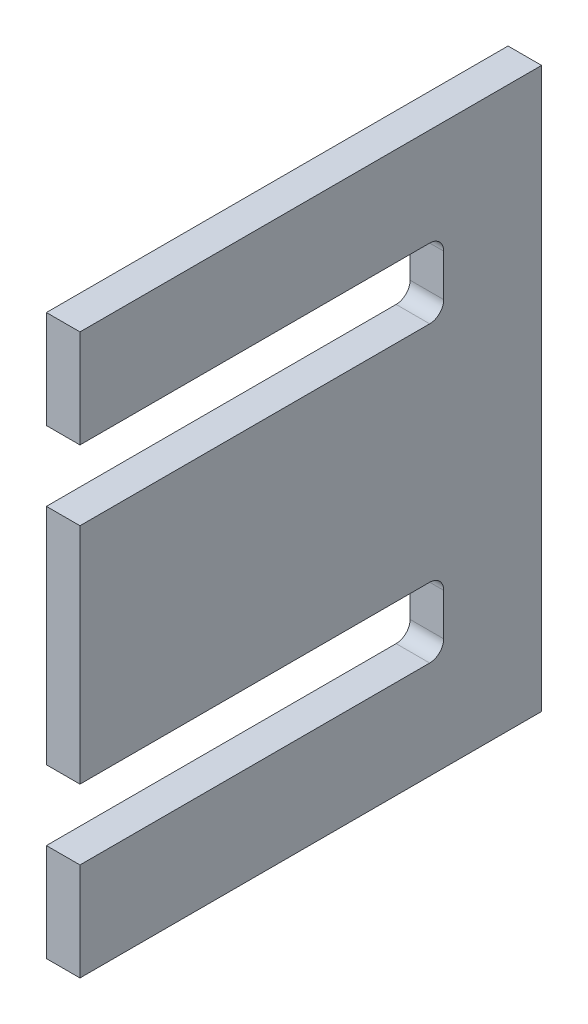
from build123d import *

# Parameters (mm, degrees)
EXTRUDE_1_DEPTH = 12


with BuildPart() as part:
    # 草图2 → 凸台-拉伸1 (new body)
    with BuildSketch(Plane.ZY.offset(140.770328303)):
        with BuildLine():
            Line((-63, -168), (-63, -153))
            ThreePointArc((-63, -153), (-61.535533906, -149.464466094), (-58, -148))
            Line((-58, -148), (67, -148))
            Line((67, -148), (67, -68))
            Line((67, -68), (-58, -68))
            ThreePointArc((-58, -68), (-61.535533906, -66.535533906), (-63, -63))
            Line((-63, -63), (-63, -48))
            ThreePointArc((-63, -48), (-61.535533906, -44.464466094), (-58, -43))
            Line((-58, -43), (67, -43))
            Line((67, -43), (67, -8))
            Line((67, -8), (-98, -8))
            Line((-98, -8), (-98, -208))
            Line((-98, -208), (67, -208))
            Line((67, -208), (67, -173))
            Line((67, -173), (-58, -173))
            ThreePointArc((-58, -173), (-61.535533906, -171.535533906), (-63, -168))
        make_face()
    extrude(amount=EXTRUDE_1_DEPTH)


solid = part.part
